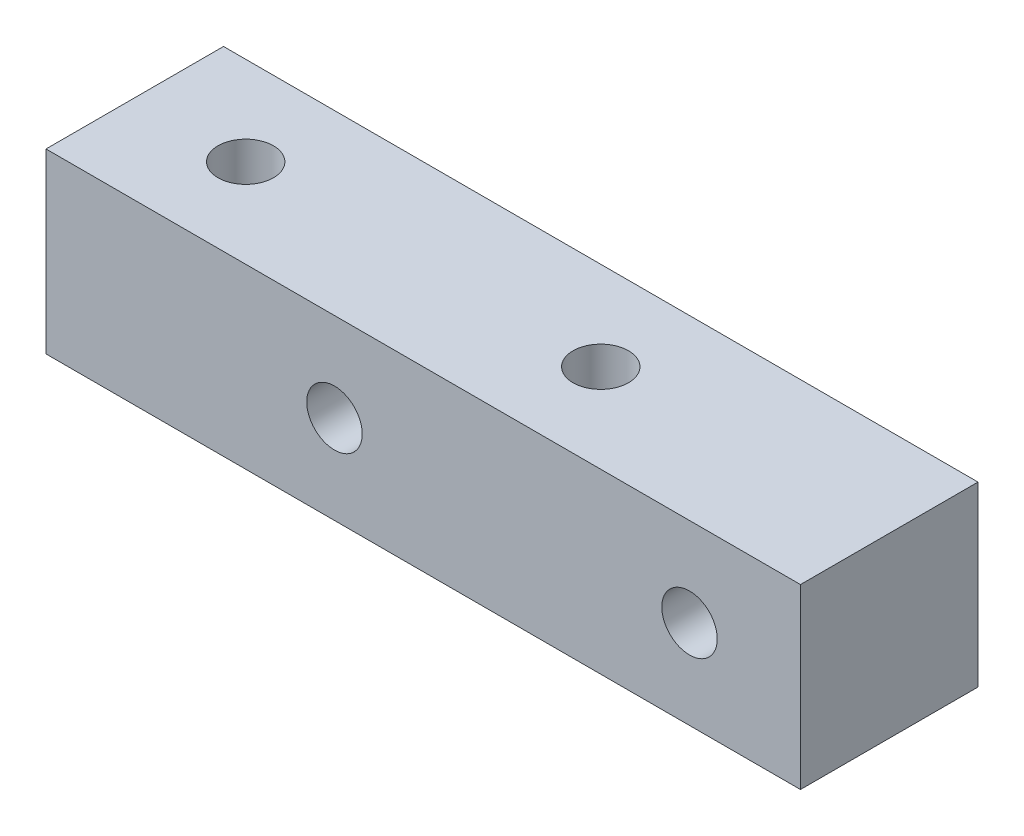
SolidWorks part; units mm, degrees
material "6061 合金"
ref_plane "前视基准面" through (0, 0, 0) normal (0, 0, 1) x (1, 0, 0)
ref_plane "上视基准面" through (0, 0, 0) normal (0, 1, 0) x (1, 0, 0)
ref_plane "右视基准面" through (0, 0, 0) normal (1, 0, 0) x (0, 0, -1)
sketch "草图1" plane through (0, 0, 0) normal (0, 1, 0) x (1, 0, 0)
  line L1 (-17, 4) -> (17, 4)
  line L2 (-17, 4) -> (-17, -4)
  line L3 (-17, -4) -> (17, -4)
  line L4 (17, 4) -> (17, -4)
  line L5 (-17, 4) -> (17, -4) construction
  line L6 (-17, -4) -> (17, 4) construction
  point P0 (0, 0)
  dimension "D1" = 34
  dimension "D2" = 8
extrude "凸台-拉伸1" add sketch "草图1" along normal blind 8
sketch "草图2" plane through (0, 8, 0) normal (0, 1, 0) x (1, 0, 0)
  line L0 (-17, 0) -> (17, 0) construction
  line L1 (-17, 4) -> (-17, -4) construction
  line L2 (17, -4) -> (17, 4) construction
  point P6 (-12, 0)
  point P7 (4, 0)
  dimension "D1" = 5
  dimension "D2" = 16
hole_wizard "M3 螺纹孔1" positions "草图2" profile "草图3" tap size "M3" standard "GB" end condition through all
sketch "草图3" plane through (4, 8, 0) normal (1, 0, 0) x (0, 0, 1)
  line L0 (0, 0) -> (0, 8)
  line L1 (0, 8) -> (1.25, 8)
  line L2 (1.25, 8) -> (1.25, 0)
  line L5 (1.25, 0) -> (0, 0)
  line L11 (0, -6.35) -> (0, 107.95) construction
  dimension "通孔螺纹孔钻头直径" = 2.5
  dimension "通孔螺纹孔钻头深度" = 8
cosmetic thread "孔螺纹线1" parameters "D2"=3
cosmetic thread "孔螺纹线2" parameters "D2"=3
sketch "草图4" plane through (0, 0, 4) normal (0, 0, 1) x (1, 0, 0)
  line L0 (-17, 4) -> (17, 4) construction
  line L1 (-17, 8) -> (-17, 0) construction
  line L2 (17, 8) -> (17, 0) construction
  point P6 (-4, 4)
  point P7 (12, 4)
  dimension "D1" = 16
  dimension "D2" = 5
hole_wizard "M3 螺纹孔2" positions "草图4" profile "草图5" tap size "M3" standard "GB" end condition through all
sketch "草图5" plane through (12, 4, 4) normal (1, 0, 0) x (0, -1, 0)
  line L0 (0, 0) -> (0, 8)
  line L1 (0, 8) -> (1.25, 8)
  line L2 (1.25, 8) -> (1.25, 0)
  line L5 (1.25, 0) -> (0, 0)
  line L11 (0, -6.35) -> (0, 107.95) construction
  dimension "通孔螺纹孔钻头直径" = 2.5
  dimension "通孔螺纹孔钻头深度" = 8
cosmetic thread "孔螺纹线3" parameters "D2"=3
cosmetic thread "孔螺纹线4" parameters "D2"=3
